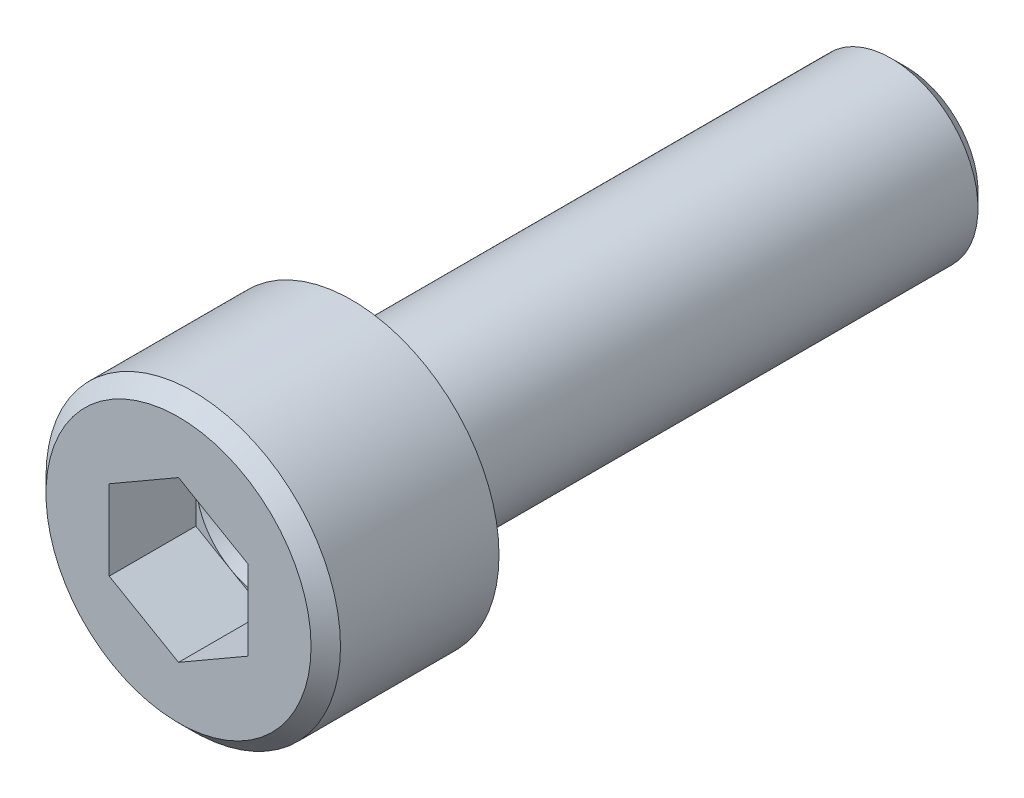
from build123d import *

# Parameters (mm, degrees)
SKETCH_1_W          = 4.25
SKETCH_1_H          = 5
SKETCH_2_R          = 2.5
EXTRUDE_1_DEPTH     = 16
CUT_EXTRUDE_1_DEPTH = 2.5
CHAMFER_1_SIZE      = 0.425


with BuildPart() as part:
    # 草图1 → 旋转1 (revolve)
    with BuildSketch(Plane(origin=(0, 0, 0), x_dir=(1, 0, 0), z_dir=(0, 1, 0))):
        with Locations((2.125, -2.5)):
            Rectangle(SKETCH_1_W, SKETCH_1_H)
    revolve(axis=Axis((0, 0, 0), (0, 0, 1)))

    # 草图2 → 凸台-拉伸1 (add)
    with BuildSketch(Plane(origin=(0, 0, 0), x_dir=(-1, 0, 0), z_dir=(0, 0, -1))):
        Circle(SKETCH_2_R)
    extrude(amount=EXTRUDE_1_DEPTH)

    # 草图3 → 切除-拉伸1 (cut)
    with BuildSketch(Plane.XY.offset(5)):
        Polygon((2, 1.154700538), (0, 2.309401077), (-2, 1.154700538), (-2, -1.154700538), (0, -2.309401077), (2, -1.154700538), align=None)
    extrude(amount=-CUT_EXTRUDE_1_DEPTH, mode=Mode.SUBTRACT)

    # 草图4 → 切除-旋转1 (revolve, cut)
    with BuildSketch(Plane.XZ, mode=Mode.PRIVATE) as cut_revolve_1_sk:
        Polygon((2, 2.5), (0, 2.5), (0, 1.345299462), align=None)
    revolve(cut_revolve_1_sk.sketch.rotate(Axis((0, 0, 2.5), (0, 0, -1)), 90), axis=Axis((0, 0, 2.5), (0, 0, -1)), mode=Mode.SUBTRACT)

    # 倒角1
    chamfer_1_edges = [part.edges().sort_by_distance(p)[0] for p in [
        (-4.25, 0, 5),
        (2.5, 0, -16),
    ]]
    chamfer(chamfer_1_edges, length=CHAMFER_1_SIZE)


solid = part.part
